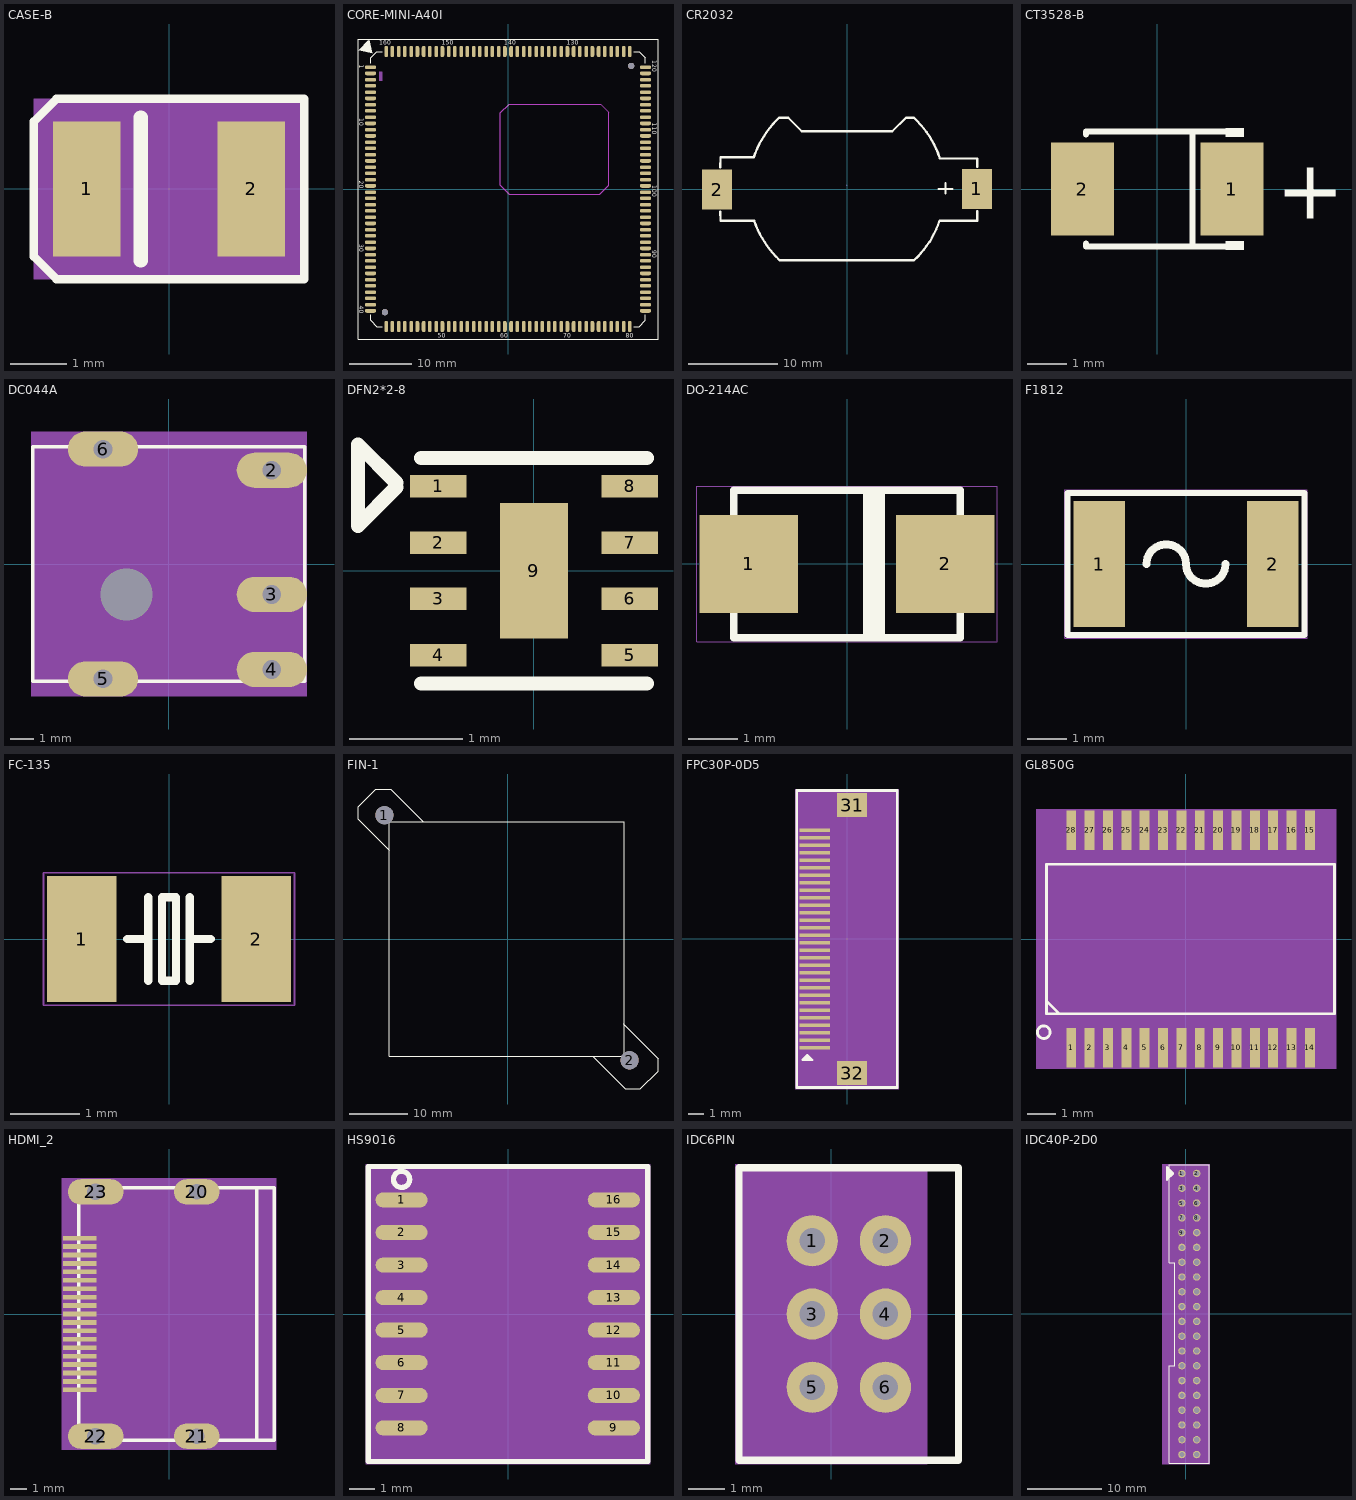
[diagram p0: the footprints below, top view; thin cyan lines are the x and y axes]
# Altium footprint library MISC84456-5.PcbLib: 85 footprints (part 2 of 6)
Each footprint in its own frame and in the unit in brackets; x right, y up, seen from the top. Pads: shape width x height; smd on the part's side, far side on the other; paste and mask are expansions set on the pad; w line width, h text height; cw(c..) or ccw(c..) is an arc to the next point about the centre after c.

## CASE-B [mm] "CASE-B"
pads (2):
  rect 1.2x2.4 smd: 1(-1.465,0) 2(1.464,0)
Top Overlay:
  lines w0.15: -2.4,-1.2 -2,-1.6 -0.1,-1.6 2.4,-1.6 2.4,1.6 -2,1.6 -2.4,1.2 -2.4,-1.2
  lines w0.254: -0.5,-1.27 -0.5,1.27
  text ".Designator" at 3,-0.325 h0.6
Mechanical 7:
  text "2" at 1.464,-0.254 h0.64
  text "1" at -1.465,-0.254 h0.64
Mechanical 8:
  region: 2.4,1.6 -2.4,1.6 -2.4,-1.6 2.4,-1.6
Mechanical 9:
  text "100uF" at 0.475,-1 h0.35

## CORE-MINI-A40I [mm] "CORE-MINI-A40I"
pads (162):
  oval 1.8x0.6 smd: 1(-22,19.5) 2(-22,18.5) 3(-22,17.5) 4(-22,16.5) 5(-22,15.5) 6(-22,14.5) 7(-22,13.5) 8(-22,12.5) 9(-22,11.5) 10(-22,10.5) 11(-22,9.5) 12(-22,8.5) 13(-22,7.5) 14(-22,6.5) 15(-22,5.5) 16(-22,4.5) 17(-22,3.5) 18(-22,2.5) 19(-22,1.5) 20(-22,0.5) 21(-22,-0.5) 22(-22,-1.5) 23(-22,-2.5) 24(-22,-3.5) 25(-22,-4.5) 26(-22,-5.5) 27(-22,-6.5) 28(-22,-7.5) 29(-22,-8.5) 30(-22,-9.5) 31(-22,-10.5) 32(-22,-11.5) 33(-22,-12.5) 34(-22,-13.5) 35(-22,-14.5) 36(-22,-15.5) 37(-22,-16.5) 38(-22,-17.5) 39(-22,-18.5) 40(-22,-19.5) 81(22,-19.5) 82(22,-18.5) 83(22,-17.5) 84(22,-16.5) 85(22,-15.5) 86(22,-14.5) 87(22,-13.5) 88(22,-12.5) 89(22,-11.5) 90(22,-10.5) 91(22,-9.5) 92(22,-8.5) 93(22,-7.5) 94(22,-6.5) 95(22,-5.5) 96(22,-4.5) 97(22,-3.5) 98(22,-2.5) 99(22,-1.5) 100(22,-0.5) 101(22,0.5) 102(22,1.5) 103(22,2.5) 104(22,3.5) 105(22,4.5) 106(22,5.5) 107(22,6.5) 108(22,7.5) 109(22,8.5) 110(22,9.5) 111(22,10.5) 112(22,11.5) 113(22,12.5) 114(22,13.5) 115(22,14.5) 116(22,15.5) 117(22,16.5) 118(22,17.5) 119(22,18.5) 120(22,19.5)
  oval 0.6x1.8 smd: 41(-19.5,-22) 42(-18.5,-22) 43(-17.5,-22) 44(-16.5,-22) 45(-15.5,-22) 46(-14.5,-22) 47(-13.5,-22) 48(-12.5,-22) 49(-11.5,-22) 50(-10.5,-22) 51(-9.5,-22) 52(-8.5,-22) 53(-7.5,-22) 54(-6.5,-22) 55(-5.5,-22) 56(-4.5,-22) 57(-3.5,-22) 58(-2.5,-22) 59(-1.5,-22) 60(-0.5,-22) 61(0.5,-22) 62(1.5,-22) 63(2.5,-22) 64(3.5,-22) 65(4.5,-22) 66(5.5,-22) 67(6.5,-22) 68(7.5,-22) 69(8.5,-22) 70(9.5,-22) 71(10.5,-22) 72(11.5,-22) 73(12.5,-22) 74(13.5,-22) 75(14.5,-22) 76(15.5,-22) 77(16.5,-22) 78(17.5,-22) 79(18.5,-22) 80(19.5,-22) 121(19.5,22) 122(18.5,22) 123(17.5,22) 124(16.5,22) 125(15.5,22) 126(14.5,22) 127(13.5,22) 128(12.5,22) 129(11.5,22) 130(10.5,22) 131(9.5,22) 132(8.5,22) 133(7.5,22) 134(6.5,22) 135(5.5,22) 136(4.5,22) 137(3.5,22) 138(2.5,22) 139(1.5,22) 140(0.5,22) 141(-0.5,22) 142(-1.5,22) 143(-2.5,22) 144(-3.5,22) 145(-4.5,22) 146(-5.5,22) 147(-6.5,22) 148(-7.5,22) 149(-8.5,22) 150(-9.5,22) 151(-10.5,22) 152(-11.5,22) 153(-12.5,22) 154(-13.5,22) 155(-14.5,22) 156(-15.5,22) 157(-16.5,22) 158(-17.5,22) 159(-18.5,22) 160(-19.5,22)
  round 1 hole 1: " "(-19.7,-19.7) " "(19.7,19.7)
Top Overlay:
  pour cut-out: -22.4,23.7 -23.7,22.4 -23.9,22.2 -21.7,21.7 -22.2,23.9
  lines w0.15: -22,-20.1 -22,-21 -21,-22 -20.1,-22 ; -22,20.1 -22,21 -21,22 -20.1,22 ; 20.1,-22 21,-22 22,-21 22,-20.1 ; 20.1,22 21,22 22,21 22,20.1 ; -24,-24 24,-24 24,24 -19.6,24 -24,24 -24,-24
  text "1" at -23.8,19.9 h0.7
  text "160" at -20.6,23.1 h0.7
  text "40" at -23.8,-18.7 h0.7
  text "10" at -23.8,11.3 h0.7
  text "20" at -23.8,1.3 h0.7
  text "30" at -23.8,-8.8 h0.7
  text "50" at -11.2,-23.8 h0.7
  text "60" at -1.2,-23.8 h0.7
  text "70" at 8.8,-23.8 h0.7
  text "80" at 18.8,-23.8 h0.7
  text "90" at 23.1,-9.8 h0.7
  text "100" at 23.1,0.6 h0.7
  text "110" at 23.1,10.6 h0.7
  text "120" at 23.1,20.6 h0.7
  text "130" at 9.4,23.1 h0.7
  text "140" at -0.6,23.1 h0.7
  text "150" at -10.6,23.1 h0.7
Keep-Out Layer:
  lines w0.025: 14.8,13.6 16.1,12.3
  lines w0.15: -1.2,0.6 -1.2,12.2 0.2,13.6 14.8,13.6 16.1,12.3 16.1,0.6 14.7,-0.8 0.2,-0.8 -1.2,0.6
Mechanical 5:
  lines w0.025: 14.8,13.6 0.2,13.6 -1.2,12.2 -1.2,0.6 0.2,-0.8 14.7,-0.8 16.1,0.6 16.1,12.3
Mechanical 7:
  text "106" at 22,6.11 h0.25
  text "15" at -22,5.906 h0.25
  text "57" at -3.5,-21.594 h0.25
  text "107" at 22,7.11 h0.25
  text "61" at 0.5,-21.594 h0.25
  text "103" at 22,3.11 h0.25
  text "53" at -7.5,-21.594 h0.25
  text "108" at 22,8.11 h0.25
  text "104" at 22,4.11 h0.25
  text "59" at -1.5,-21.594 h0.25
  text "1" at -22,19.703 h0.25
  text "55" at -5.5,-21.594 h0.25
  text "160" at -19.5,22.61 h0.25
  text "56" at -4.5,-21.594 h0.25
  text "159" at -18.5,22.61 h0.25
  text "105" at 22,5.11 h0.25
  text "60" at -0.5,-21.594 h0.25
  text "158" at -17.5,22.61 h0.25
  text "58" at -2.5,-21.594 h0.25
  text "52" at -8.5,-21.594 h0.25
  text "54" at -6.5,-21.594 h0.25
  text "136" at 4.5,22.61 h0.25
  text "133" at 7.5,22.61 h0.25
  text "126" at 14.5,22.61 h0.25
  text "125" at 15.5,22.61 h0.25
  text "128" at 12.5,22.61 h0.25
  text "131" at 9.5,22.61 h0.25
  text "132" at 8.5,22.61 h0.25
  text "127" at 13.5,22.61 h0.25
  text "124" at 16.5,22.61 h0.25
  text "130" at 10.5,22.61 h0.25
  text "129" at 11.5,22.61 h0.25
  text "137" at 3.5,22.61 h0.25
  text "142" at -1.5,22.61 h0.25
  text "141" at -0.5,22.61 h0.25
  text "134" at 6.5,22.61 h0.25
  text "14" at -22,6.906 h0.25
  text "138" at 2.5,22.61 h0.25
  text "13" at -22,7.906 h0.25
  text "139" at 1.5,22.61 h0.25
  text "145" at -4.5,22.61 h0.25
  text "12" at -22,8.906 h0.25
  text "140" at 0.5,22.61 h0.25
  text "2" at -22,18.703 h0.25
  text "77" at 16.5,-21.594 h0.25
  text "11" at -22,9.906 h0.25
  text "79" at 18.5,-21.594 h0.25
  text "75" at 14.5,-21.594 h0.25
  text "135" at 5.5,22.61 h0.25
  text "3" at -22,17.703 h0.25
  text "21" at -22,-0.094 h0.25
  text "76" at 15.5,-21.594 h0.25
  text "116" at 22,16.11 h0.25
  text "151" at -10.5,22.61 h0.25
  text "80" at 19.5,-21.594 h0.25
  text "150" at -9.5,22.61 h0.25
  text "17" at -22,3.906 h0.25
  text "66" at 5.5,-21.594 h0.25
  text "41" at -19.5,-21.594 h0.25
  text "34" at -22,-13.094 h0.25
  text "28" at -22,-7.094 h0.25
  text "37" at -22,-16.094 h0.25
  text "64" at 3.5,-21.594 h0.25
  text "29" at -22,-8.094 h0.25
  text "32" at -22,-11.094 h0.25
  text "153" at -12.5,22.61 h0.25
  text "63" at 2.5,-21.594 h0.25
  text "70" at 9.5,-21.594 h0.25
  text "18" at -22,2.906 h0.25
  text "42" at -18.5,-21.594 h0.25
  text "30" at -22,-9.094 h0.25
  text "157" at -16.5,22.61 h0.25
  text "62" at 1.5,-21.594 h0.25
  text "16" at -22,4.906 h0.25
  text "67" at 6.5,-21.594 h0.25
  text "154" at -13.5,22.61 h0.25
  text "68" at 7.5,-21.594 h0.25
  text "25" at -22,-4.094 h0.25
  text "31" at -22,-10.094 h0.25
  text "69" at 8.5,-21.594 h0.25
  text "20" at -22,0.906 h0.25
  text "71" at 10.5,-21.594 h0.25
  text "74" at 13.5,-21.594 h0.25
  text "65" at 4.5,-21.594 h0.25
  text "35" at -22,-14.094 h0.25
  text "155" at -14.5,22.61 h0.25
  text "110" at 22,10.11 h0.25
  text "33" at -22,-12.094 h0.25
  text "36" at -22,-15.094 h0.25
  text "117" at 22,17.11 h0.25
  text "111" at 22,11.11 h0.25
  text "73" at 12.5,-21.594 h0.25
  text "121" at 19.5,22.61 h0.25
  text "119" at 22,19.11 h0.25
  text "72" at 11.5,-21.594 h0.25
  text "8" at -22,12.703 h0.25
  text "118" at 22,18.11 h0.25
  text "44" at -16.5,-21.594 h0.25
  text "9" at -22,11.703 h0.25
  text "45" at -15.5,-21.594 h0.25
  text "112" at 22,12.11 h0.25
  text "109" at 22,9.11 h0.25
  text "46" at -14.5,-21.594 h0.25
  text "114" at 22,14.11 h0.25
  text "47" at -13.5,-21.594 h0.25
  text "51" at -9.5,-21.594 h0.25
  text "122" at 18.5,22.61 h0.25
  text "19" at -22,1.906 h0.25
  text "7" at -22,13.703 h0.25
  text "48" at -12.5,-21.594 h0.25
  text "144" at -3.5,22.61 h0.25
  text "49" at -11.5,-21.594 h0.25
  text "113" at 22,13.11 h0.25
  text "50" at -10.5,-21.594 h0.25
  text "81" at 22,-19.094 h0.25
  text "120" at 22,20.11 h0.25
  text "102" at 22,2.11 h0.25
  text "99" at 22,-1.094 h0.25
  text "152" at -11.5,22.61 h0.25
  text "6" at -22,14.703 h0.25
  text "143" at -2.5,22.61 h0.25
  text "100" at 22,0.11 h0.25
  text "97" at 22,-3.094 h0.25
  text "123" at 17.5,22.61 h0.25
  text "156" at -15.5,22.61 h0.25
  text "101" at 22,1.11 h0.25
  text "98" at 22,-2.094 h0.25
  text "10" at -22,10.906 h0.25
  text "149" at -8.5,22.61 h0.25
  text "85" at 22,-15.094 h0.25
  text "93" at 22,-7.094 h0.25
  text "86" at 22,-14.094 h0.25
  text "88" at 22,-12.094 h0.25
  text "83" at 22,-17.094 h0.25
  text "90" at 22,-10.094 h0.25
  text "94" at 22,-6.094 h0.25
  text "87" at 22,-13.094 h0.25
  text "96" at 22,-4.094 h0.25
  text "89" at 22,-11.094 h0.25
  text "84" at 22,-16.094 h0.25
  text "91" at 22,-9.094 h0.25
  text "92" at 22,-8.094 h0.25
  text "5" at -22,15.703 h0.25
  text "4" at -22,16.703 h0.25
  text "23" at -22,-2.094 h0.25
  text "22" at -22,-1.094 h0.25
  text "43" at -17.5,-21.594 h0.25
  text "40" at -22,-19.094 h0.25
  text "27" at -22,-6.094 h0.25
  text "26" at -22,-5.094 h0.25
  text "148" at -7.5,22.61 h0.25
  text "82" at 22,-18.094 h0.25
  text "24" at -22,-3.094 h0.25
  text "147" at -6.5,22.61 h0.25
  text "146" at -5.5,22.61 h0.25
  text "38" at -22,-17.094 h0.25
  text "115" at 22,15.11 h0.25
  text "39" at -22,-18.094 h0.25
  text "78" at 17.5,-21.594 h0.25
  text "95" at 22,-5.094 h0.25
Mechanical 8:
  region: -20.1,18.75 -20.6,18.75 -20.6,17.3 -20.1,17.3 -20.1,17.8

## CR2032 [mm]
pads (2):
  rect 3.4x4.5 smd: 1(14.575,0.032) 2(-14.575,-0.032)
Top Overlay:
  lines w0.254: -14.224,-2.508 -14.201,-3.524 -10.85,-3.524 -10.414,-3.524 ccw(c0,0.032) -7.571,-7.954 7.52,-7.954 ; -14.224,2.445 -14.201,3.588 -10.85,3.588 -10.467,3.588 ; -10.467,3.563 cw(c0,0.032) -7.618,8.032 -6.603,8.032 -5.08,6.509 5.08,6.509 6.608,8.037 7.491,8.037 cw(c0,0.032) 10.414,3.461 14.605,3.461 14.605,2.513 ; 7.52,-7.968 ccw(c0,0.032) 10.391,-3.516 ; 10.287,0.032 11.811,0.032 ; 10.391,-3.524 11.15,-3.524 14.628,-3.524 ; 11.049,-0.476 11.049,0.667 ; 14.605,-3.524 14.605,-2.449
Mechanical 15:
  lines w0.003: -0.025,0.458 0.025,0.509

## CT3528-B [mm]
pads (2):
  rect 1.607x2.376 smd: 1(1.911,0) 2(-1.911,0)
Top Overlay:
  region: 1.75,-1.552 1.75,-1.34 2.207,-1.34 2.207,-1.552
  region: 1.75,1.552 1.75,1.34 2.207,1.34 2.207,1.552
  lines w0.152: -1.826,-1.391 -1.826,-1.476 1.826,-1.476 ; -1.826,1.391 -1.826,1.476 1.826,1.476 ; 0.904,-1.476 0.904,1.476
  text "+" at 3.048,-0.762 h1.52
Mechanical 5:
  region: 1.98,-1.1 1.98,1.1 1.28,1.1 1.28,-1.1
  region: -1.98,-1.1 -1.98,1.1 -1.28,1.1 -1.28,-1.1

## DC044A [mm] "DC044A"
pads (6):
  oval 3x1.5 hole 0.8: 2(4.387,4) 3(4.387,-1.3) 4(4.387,-4.5) 5(-2.812,-4.9) 6(-2.812,4.9)
  round 2 hole 2.2: " "(-1.812,-1.3)
Top Overlay:
  lines w0.15: -5.813,-5 5.788,-5 5.788,5 -5.813,5 -5.813,-5
Mechanical 7:
  text "3" at 4.387,-1.364 h0.08
  text "2" at 4.387,3.936 h0.08
  text "5" at -2.812,-4.964 h0.08
  text "6" at -2.812,4.836 h0.08
  text "4" at 4.387,-4.564 h0.08
Mechanical 8:
  region: -5.887,-5.65 5.888,-5.65 5.888,5.65 -5.887,5.65
Mechanical 9:
  text "DC_5V" at 1.062,-1.125 h0.35
  text ".Designator" at -3.213,-0.025 h0.35

## DFN2*2-8 [mm]
pads (9):
  rect 0.5x0.2 smd: 1(-0.85,0.75) 2(-0.85,0.25) 3(-0.85,-0.25) 4(-0.85,-0.75) 5(0.85,-0.75) 6(0.85,-0.25) 7(0.85,0.25) 8(0.85,0.75)
  rect 0.6x1.2 smd: 9(0,0)
Top Overlay:
  lines w0.127: -1.22,0.74 -1.56,0.4 -1.56,1.12 -1.22,0.78 ; -1,-1 1,-1 ; -1,1 1,1

## DO-214AC [mm] "DO-214AC"
pads (2):
  rect 1.999x1.999 smd: 1(-1.999,0) 2(1.999,0)
Top Overlay:
  lines w0.152: 0.399,-1.501 0.399,1.501 ; 0.551,-1.501 0.551,1.501 ; 0.701,-1.501 0.701,1.501 ; -2.301,-1.501 -2.301,1.501 2.301,1.501 2.301,-1.501 -2.301,-1.501
  text ".Designator" at -4.425,-0.15 h0.6
Mechanical 7:
  text "2" at 1.745,0 h0.64
  text "1" at -2.253,0 h0.64
Mechanical 8:
  lines w0.025: -3.051,-1.577 3.05,-1.577 3.05,1.577 -3.051,1.577 -3.051,-1.577
Mechanical 9:
  text "SMAJ16A" at -1.275,-0.2 h0.35

## F1812 [mm] "F1812"
pads (2):
  rect 1.3x3.2 smd: 1(-2.2,0) 2(2.2,0)
Top Overlay:
  lines w0.15: -3,-1.8 -3,1.8 2.8,1.8 3,1.8 3,-1.8 -3,-1.8
  lines w0.2: -1,0 cw(c-0.5,0) 0,0 ccw(c0.5,0) 1,0
  text ".Designator" at -4.275,-0.4 h0.6
Mechanical 7:
  text "1" at -2.399,0 h0.5
  text "2" at 2,0 h0.5
Mechanical 8:
  lines w0.025: -3.075,-1.875 -3.075,1.875 3.075,1.875 3.075,-1.875 -3.075,-1.875
Mechanical 9:
  text "FS-1.5A-1812" at -1.825,-0.175 h0.35

## FC-135 [mm] "FC-135"
pads (2):
  rect 1x1.8 smd: 1(-1.25,0) 2(1.25,0)
Top Overlay:
  lines w0.12: -0.6,0 -0.3,0 ; -0.3,-0.6 -0.3,0.6 ; 0.3,-0.6 0.3,0.6 ; 0.3,0 0.6,0 ; -0.1,-0.6 0.1,-0.6 0.1,0.6 -0.1,0.6 -0.1,-0.6
  text ".Designator" at 2.125,0.675 h0.6
Mechanical 7:
  text "2" at 0.69,0 h0.7
  text "1" at -1.81,0 h0.7
Mechanical 8:
  lines w0.025: -1.8,-0.95 1.8,-0.95 1.8,0.95 -1.8,0.95 -1.8,-0.95
Mechanical 9:
  text "32.768K" at -1.075,-0.225 h0.35

## FIN-1 [mm] "FIN-1"
pads (2):
  round 3.1 hole 3.1: 1(-21.075,21.113) 2(20.725,-20.687)
Top Overlay:
  lines w0.15: -20.275,15.112 -25.575,20.413 -25.575,22.513 -22.575,25.513 -19.975,25.513 -14.475,20.013 ; 14.45,-19.987 19.975,-25.512 22.575,-25.512 25.575,-22.512 25.575,-20.412 19.725,-14.562 19.725,-14.487 ; -20.275,-19.987 19.725,-19.987 19.725,20.013 -20.275,20.013 -20.275,-19.987
  text ".Designator" at -22.113,19.039 h0.6
Mechanical 7:
  text "1" at -20.895,20.933 h0.64
  text "2" at 20.905,-20.867 h0.64

## FPC30P-0D5 [mm] "FPC30P-0D5"
pads (32):
  rect 2x0.25 smd: 1(-2.15,-7.25) 2(-2.15,-6.749) 3(-2.15,-6.249) 4(-2.15,-5.751) 5(-2.15,-5.251) 6(-2.15,-4.75) 7(-2.15,-4.25) 8(-2.15,-3.75) 9(-2.15,-3.249) 10(-2.15,-2.749) 11(-2.15,-2.251) 12(-2.15,-1.751) 13(-2.15,-1.25) 14(-2.15,-0.75) 15(-2.15,-0.25) 16(-2.15,0.251) 17(-2.15,0.751) 18(-2.15,1.249) 19(-2.15,1.749) 20(-2.15,2.25) 21(-2.15,2.75) 22(-2.15,3.251) 23(-2.15,3.751) 24(-2.15,4.249) 25(-2.15,4.749) 26(-2.15,5.249) 27(-2.15,5.75) 28(-2.15,6.25) 29(-2.15,6.751) 30(-2.15,7.251)
  rect 2x1.6 smd: 31(0.35,8.919) 32(0.35,-8.949)
Top Overlay:
  lines w0.152: -2.819,-7.96 -2.489,-7.96 ; -2.74,-7.861 -2.55,-7.861 ; -2.649,-7.739 -2.324,-8.064 -2.969,-8.064 -2.646,-7.742
  lines w0.2: -3.35,-9.9 3.35,-9.9 3.35,9.9 0.95,9.9 -3.35,9.9 -3.35,-9.9
  text ".Designator" at 6.825,-1.075 h0.6
Mechanical 7:
  text "7" at -2.11,-4.25 h0.1
  text "26" at -2.07,5.249 h0.1
  text "17" at -2.07,0.751 h0.1
  text "14" at -2.07,-0.75 h0.1
  text "30" at -2.07,7.251 h0.1
  text "20" at -2.07,2.25 h0.1
  text "8" at -2.11,-3.75 h0.1
  text "6" at -2.11,-4.75 h0.1
  text "29" at -2.07,6.751 h0.1
  text "27" at -2.07,5.75 h0.1
  text "23" at -2.07,3.751 h0.1
  text "15" at -2.07,-0.25 h0.1
  text "24" at -2.07,4.249 h0.1
  text "21" at -2.07,2.75 h0.1
  text "18" at -2.07,1.249 h0.1
  text "9" at -2.11,-3.249 h0.1
  text "12" at -2.07,-1.751 h0.1
  text "11" at -2.07,-2.251 h0.1
  text "3" at -2.11,-6.249 h0.1
  text "5" at -2.11,-5.251 h0.1
  text "1" at -2.11,-7.25 h0.1
  text "31" at 0.43,8.919 h0.1
  text "22" at -2.07,3.251 h0.1
  text "25" at -2.07,4.749 h0.1
  text "28" at -2.07,6.25 h0.1
  text "32" at 0.43,-8.949 h0.1
  text "19" at -2.07,1.749 h0.1
  text "4" at -2.11,-5.751 h0.1
  text "2" at -2.11,-6.749 h0.1
  text "13" at -2.07,-1.25 h0.1
  text "16" at -2.07,0.251 h0.1
  text "10" at -2.07,-2.749 h0.1
Mechanical 8:
  region: -3.45,-10 3.45,-10 3.45,10 -3.45,10

## GL850G [mm] "GL850G"
pads (28):
  rect 0.35x1.4 smd: 1(-4.063,-3.85) 2(-3.413,-3.85) 3(-2.763,-3.85) 4(-2.113,-3.85) 5(-1.463,-3.85) 6(-0.813,-3.85) 7(-0.163,-3.85) 8(0.487,-3.85) 9(1.137,-3.85) 10(1.787,-3.85) 11(2.437,-3.85) 12(3.087,-3.85) 13(3.737,-3.85) 14(4.387,-3.85) 15(4.387,3.85) 16(3.737,3.85) 17(3.087,3.85) 18(2.437,3.85) 19(1.787,3.85) 20(1.137,3.85) 21(0.487,3.85) 22(-0.163,3.85) 23(-0.813,3.85) 24(-1.463,3.85) 25(-2.113,3.85) 26(-2.763,3.85) 27(-3.413,3.85) 28(-4.063,3.85)
Top Overlay:
  circle w0.1: c-5.038,-3.3 r0.224
  lines w0.1: -4.938,-2.2 -4.538,-2.6 ; -4.938,-2.65 -4.938,2.65 5.262,2.65 5.262,-2.65 -4.938,-2.65
  text ".Designator" at -5.738,-2.4 h0.6
Mechanical 7:
  text "16" at 3.737,3.342 h0.64
  text "24" at -1.463,3.342 h0.64
  text "5" at -1.463,-4.104 h0.64
  text "1" at -4.063,-4.104 h0.64
  text "10" at 1.787,-4.358 h0.64
  text "26" at -2.763,3.342 h0.64
  text "4" at -2.113,-4.104 h0.64
  text "21" at 0.487,3.342 h0.64
  text "6" at -0.813,-4.104 h0.64
  text "7" at -0.163,-4.104 h0.64
  text "17" at 3.087,3.342 h0.64
  text "13" at 3.737,-4.358 h0.64
  text "25" at -2.113,3.342 h0.64
  text "18" at 2.437,3.342 h0.64
  text "23" at -0.813,3.342 h0.64
  text "27" at -3.413,3.342 h0.64
  text "11" at 2.437,-4.358 h0.64
  text "8" at 0.487,-4.104 h0.64
  text "12" at 3.087,-4.358 h0.64
  text "3" at -2.763,-4.104 h0.64
  text "2" at -3.413,-4.104 h0.64
  text "28" at -4.063,3.342 h0.64
  text "9" at 1.137,-4.104 h0.64
  text "15" at 4.387,3.342 h0.64
  text "14" at 4.387,-4.358 h0.64
  text "20" at 1.137,3.342 h0.64
  text "22" at -0.163,3.342 h0.64
  text "19" at 1.787,3.342 h0.64
Mechanical 8:
  region: -5.312,-4.6 5.312,-4.6 5.312,4.6 -5.312,4.6
Mechanical 9:
  text "GL850G" at -3.838,-1.4 h0.35

## HDMI_2 [mm] "HDMI_2"
pads (23):
  rect 2x0.28 smd: 1(-5.301,4.5) 2(-5.301,4) 3(-5.301,3.5) 4(-5.301,3) 5(-5.301,2.5) 6(-5.301,2) 7(-5.301,1.5) 8(-5.301,1) 9(-5.301,0.5) 10(-5.301,0) 11(-5.301,-0.5) 12(-5.301,-1) 13(-5.301,-1.5) 14(-5.301,-2) 15(-5.301,-2.5) 16(-5.301,-3) 17(-5.301,-3.5) 18(-5.301,-4) 19(-5.301,-4.5)
  oval 2.7x1.5 hole 0.9: 20(1.649,7.25) 21(1.649,-7.25)
  oval 3.3x1.5 hole 1: 22(-4.351,-7.25) 23(-4.351,7.25)
Top Overlay:
  lines w0.203: 5.199,-7.5 5.199,7.5 ; -5.351,-7.5 6.249,-7.5 6.249,7.5 -5.351,7.5 -5.351,-7.5
Mechanical 7:
  text "15" at -5.301,-1.992 h0.64
  text "3" at -5.301,3.754 h0.64
  text "13" at -5.301,-0.992 h0.64
  text "10" at -5.301,0.508 h0.64
  text "7" at -5.301,1.754 h0.64
  text "18" at -5.301,-3.492 h0.64
  text "19" at -5.301,-3.992 h0.64
  text "1" at -5.301,4.754 h0.64
  text "12" at -5.301,-0.492 h0.64
  text "9" at -5.301,0.754 h0.64
  text "16" at -5.301,-2.492 h0.64
  text "6" at -5.301,2.254 h0.64
  text "4" at -5.301,3.254 h0.64
  text "14" at -5.301,-1.492 h0.64
  text "20" at 1.649,7.758 h0.64
  text "21" at 1.649,-6.742 h0.64
  text "22" at -4.351,-6.742 h0.64
  text "23" at -4.351,7.758 h0.64
  text "5" at -5.301,2.754 h0.64
  text "2" at -5.301,4.254 h0.64
  text "17" at -5.301,-2.992 h0.64
  text "11" at -5.301,0.008 h0.64
  text "8" at -5.301,1.254 h0.64
Mechanical 8:
  region: -6.351,-8.05 6.351,-8.05 6.351,8.05 -6.351,8.05
Mechanical 9:
  text ".Designator" at 2.999,0.675 h0.35

## HS9016 [mm] "HS9016"
pads (16):
  oval 2.032x0.584 smd: 1(-4.15,4.45) 2(-4.15,3.18) 3(-4.15,1.91) 4(-4.15,0.64) 5(-4.15,-0.63) 6(-4.15,-1.9) 7(-4.15,-3.17) 8(-4.15,-4.44) 9(4.125,-4.44) 10(4.125,-3.17) 11(4.125,-1.9) 12(4.125,-0.63) 13(4.125,0.64) 14(4.125,1.91) 15(4.125,3.18) 16(4.125,4.45)
Top Overlay:
  circle w0.2: c-4.15,5.25 r0.316
  lines w0.2: -5.45,-5.75 -5.45,-4.25 -5.45,5.75 5.45,5.75 5.45,-5.75 -5.45,-5.75
Mechanical 7:
  text "11" at 4.531,-1.9 h0.51
  text "14" at 4.531,1.91 h0.51
  text "9" at 4.328,-4.44 h0.51
  text "16" at 4.531,4.45 h0.51
  text "12" at 4.531,-0.63 h0.51
  text "7" at -3.947,-3.17 h0.51
  text "4" at -3.947,0.64 h0.51
  text "2" at -3.947,3.18 h0.51
  text "13" at 4.531,0.64 h0.51
  text "1" at -3.947,4.45 h0.51
  text "8" at -3.947,-4.44 h0.51
  text "5" at -3.947,-0.63 h0.51
  text "15" at 4.531,3.18 h0.51
  text "6" at -3.947,-1.9 h0.51
  text "10" at 4.531,-3.17 h0.51
  text "3" at -3.947,1.91 h0.51
Mechanical 8:
  region: 5.55,-4.796 5.55,4.806 5.55,5.85 -5.55,5.85 -5.55,4.806 -5.55,-4.796 -5.55,-5.85 5.55,-5.85
Mechanical 9:
  text ".Designator" at 0.645,0.025 h0.35
Mechanical 10:
  pour cut-out: 5.55,-4.796 5.55,4.806 5.55,5.85 -5.55,5.85 -5.55,4.806 -5.55,-4.796 -5.55,-5.85 5.55,-5.85

## IDC6PIN [mm] "IDC6PIN"
pads (6):
  round 1.4 hole 0.7: 1(-0.525,2) 2(1.475,2) 3(-0.525,0) 4(1.475,0) 5(-0.525,-2) 6(1.475,-2)
Top Overlay:
  lines w0.2: -2.525,-4 -2.525,-2 -2.525,-1 -2.525,4 3.475,4 3.475,-2 3.475,-4 -2.525,-4
Mechanical 7:
  text "3" at -0.525,-0.254 h0.64
  text "1" at -0.525,1.746 h0.64
  text "6" at 1.475,-2.254 h0.64
  text "4" at 1.475,-0.254 h0.64
  text "2" at 1.475,1.746 h0.64
  text "5" at -0.525,-2.254 h0.64
Mechanical 8:
  region: -2.625,-4.1 2.625,-4.1 2.625,4.1 -2.625,4.1
Mechanical 9:
  text ".Designator" at -1.775,-1.1 h0.35

## IDC40P-2D0 [mm] "IDC40P-2D0"
pads (40):
  round 1 hole 0.7: 1(-0.549,19) 2(1.451,19) 3(-0.549,17) 4(1.451,17) 5(-0.549,15) 6(1.451,15) 7(-0.549,13) 8(1.451,13) 9(-0.549,11) 10(1.451,11) 11(-0.549,9) 12(1.451,9) 13(-0.549,7) 14(1.451,7) 15(-0.549,5) 16(1.451,5) 17(-0.549,3) 18(1.451,3) 19(-0.549,1) 20(1.451,1) 21(-0.549,-1) 22(1.451,-1) 23(-0.549,-3) 24(1.451,-3) 25(-0.549,-5) 26(1.451,-5) 27(-0.549,-7) 28(1.451,-7) 29(-0.549,-9) 30(1.451,-9) 31(-0.549,-11) 32(1.451,-11) 33(-0.549,-13) 34(1.451,-13) 35(-0.549,-15) 36(1.451,-15) 37(-0.549,-17) 38(1.451,-17) 39(-0.549,-19) 40(1.451,-19)
Top Overlay:
  lines w0.15: -2.249,-20.2 3.151,-20.2 3.151,20.2 -2.249,20.2 -2.249,6.9 -1.549,6.9 -1.549,-7 -2.249,-7 -2.249,-20.2
  lines w0.254: -2.324,18.425 -2.324,19.625 ; -2.124,18.625 -2.124,19.325 ; -1.924,18.925 -1.924,19.125 ; -1.749,18.95 -2.574,18.125 -2.574,19.875 -1.724,19.025
Mechanical 7:
  text "24" at 1.981,-4.116 h0.64
  text "20" at 1.451,0.492 h0.64
  text "30" at 1.981,-10.116 h0.64
  text "22" at 1.981,-2.116 h0.64
  text "28" at 1.981,-8.116 h0.64
  text "23" at -0.019,-4.116 h0.64
  text "19" at -0.549,0.492 h0.64
  text "21" at -0.019,-2.116 h0.64
  text "29" at -0.019,-10.116 h0.64
  text "27" at -0.019,-8.116 h0.64
  text "11" at -0.549,8.492 h0.64
  text "15" at -0.549,4.492 h0.64
  text "18" at 1.451,2.492 h0.64
  text "7" at -0.549,12.746 h0.64
  text "17" at -0.549,2.492 h0.64
  text "12" at 1.451,8.492 h0.64
  text "9" at -0.549,10.746 h0.64
  text "10" at 1.451,10.492 h0.64
  text "8" at 1.451,12.746 h0.64
  text "16" at 1.451,4.492 h0.64
  text "40" at 1.981,-20.116 h0.64
  text "39" at -0.019,-20.116 h0.64
  text "38" at 1.981,-18.116 h0.64
  text "37" at -0.019,-18.116 h0.64
  text "33" at -0.019,-14.116 h0.64
  text "36" at 1.981,-16.116 h0.64
  text "35" at -0.019,-16.116 h0.64
  text "34" at 1.981,-14.116 h0.64
  text "3" at -0.549,16.746 h0.64
  text "2" at 1.451,18.746 h0.64
  text "1" at -0.549,18.746 h0.64
  text "32" at 1.981,-12.116 h0.64
  text "25" at -0.019,-6.116 h0.64
  text "31" at -0.019,-12.116 h0.64
  text "5" at -0.549,14.746 h0.64
  text "13" at -0.549,6.492 h0.64
  text "14" at 1.451,6.492 h0.64
  text "6" at 1.451,14.746 h0.64
  text "26" at 1.981,-6.116 h0.64
  text "4" at 1.451,16.746 h0.64
Mechanical 8:
  region: -3.226,-20.275 3.226,-20.275 3.226,20.275 -3.226,20.275
Mechanical 9:
  text ".Designator" at 0.801,-2.525 h0.35